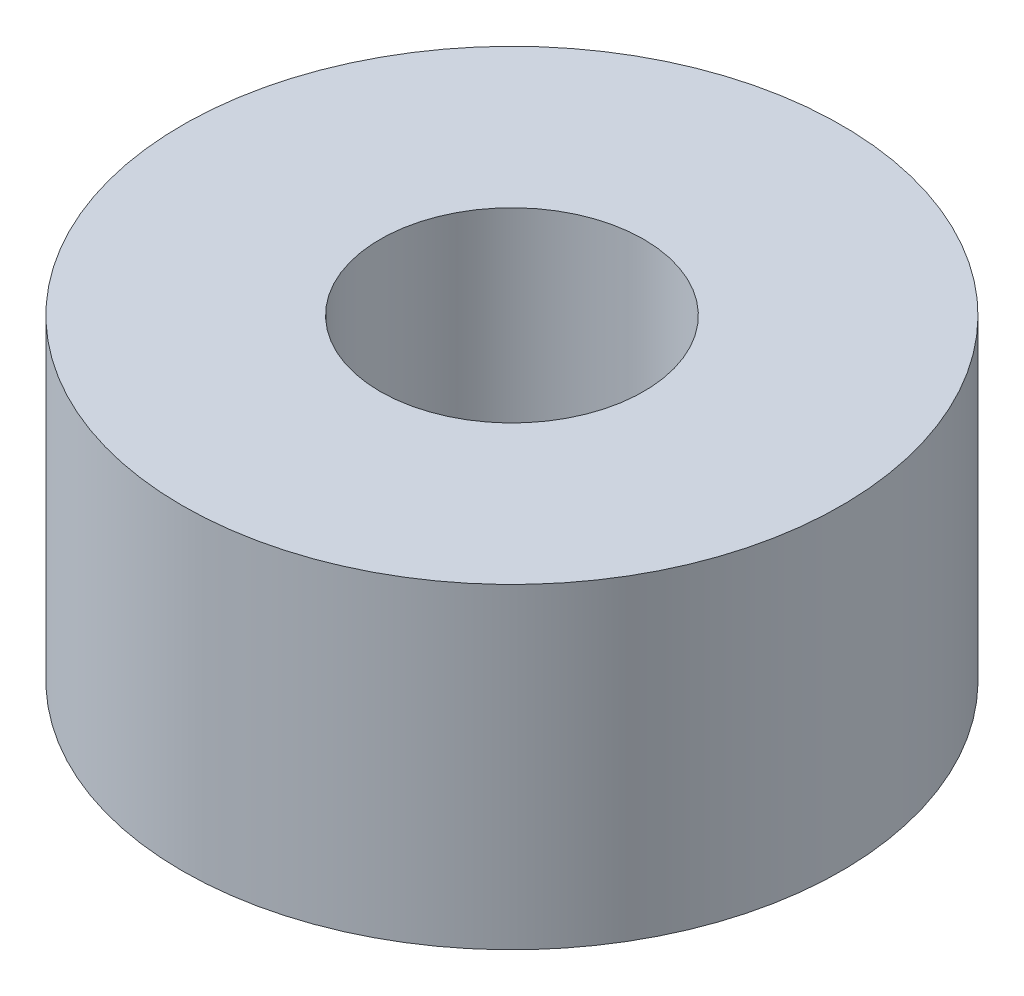
SolidWorks part; units mm, degrees
ref_plane "Front Plane" through (0, 0, 0) normal (0, 0, 1) x (1, 0, 0)
ref_plane "Top Plane" through (0, 0, 0) normal (0, 1, 0) x (1, 0, 0)
ref_plane "Right Plane" through (0, 0, 0) normal (1, 0, 0) x (0, 0, -1)
sketch "Sketch1" plane through (0, 0, 0) normal (0, 1, 0) x (1, 0, 0)
  circle A0 centre (0, 0) radius 125
  circle A1 centre (0, 0) radius 50
  dimension "D1" = 250
  dimension "D2" = 100
extrude "Boss-Extrude1" add sketch "Sketch1" along normal mid plane 120
